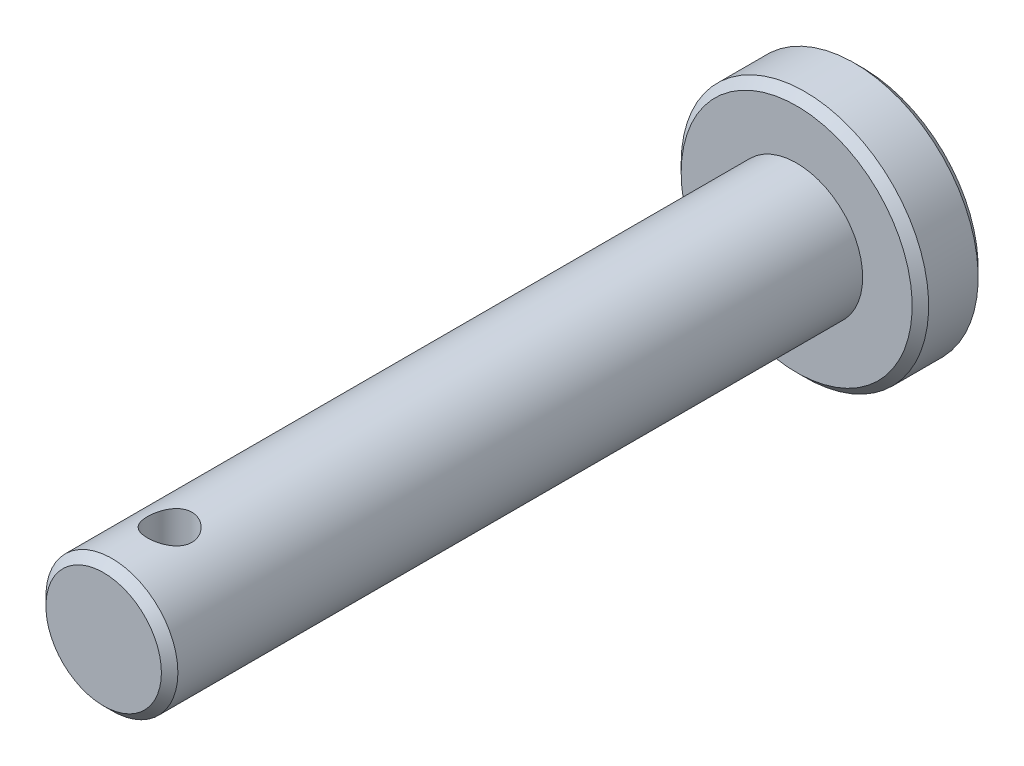
from build123d import *

# Parameters (mm, degrees)
SKETCH1_R               = 4
BOSS_EXTRUDE1_DEPTH     = 42
SKETCH2_R               = 7.5
BOSS_EXTRUDE2_DEPTH     = 4
CUT_EXTRUDE1_DEPTH      = 44.318587235
CUT_EXTRUDE1_DEPTH_BACK = 44.318587235
SKETCH3_R               = 1.35
CHAMFER1_SIZE           = 0.5


with BuildPart() as part:
    # Sketch1 → Boss-Extrude1 (new body)
    with BuildSketch(Plane.XY):
        with Locations(Location((0, 0, 0), (0, 0, 180))):
            Circle(SKETCH1_R)
    extrude(amount=BOSS_EXTRUDE1_DEPTH)

    # Sketch2 → Boss-Extrude2 (add)
    with BuildSketch(Plane(origin=(0, 0, 0), x_dir=(-1, 0, 0), z_dir=(0, 0, -1))):
        Circle(SKETCH2_R)
    extrude(amount=BOSS_EXTRUDE2_DEPTH)

    # Sketch3 → Cut-Extrude1 (cut, two sides: drawn at the far end of the back side and taken through both)
    with BuildSketch(Plane(origin=(0, 0, 0), x_dir=(1, 0, 0), z_dir=(0, 1, 0)).offset(-CUT_EXTRUDE1_DEPTH_BACK)):
        with Locations(Location((0, -38, 0), (0, 0, 270))):
            Circle(SKETCH3_R)
    extrude(amount=CUT_EXTRUDE1_DEPTH + CUT_EXTRUDE1_DEPTH_BACK, mode=Mode.SUBTRACT)

    # Chamfer1
    chamfer1_edges = [part.edges().sort_by_distance(p)[0] for p in [
        (4, 0, 42),
        (7.5, 0, 0),
        (7.5, 0, -4),
    ]]
    chamfer(chamfer1_edges, length=CHAMFER1_SIZE)


solid = part.part
